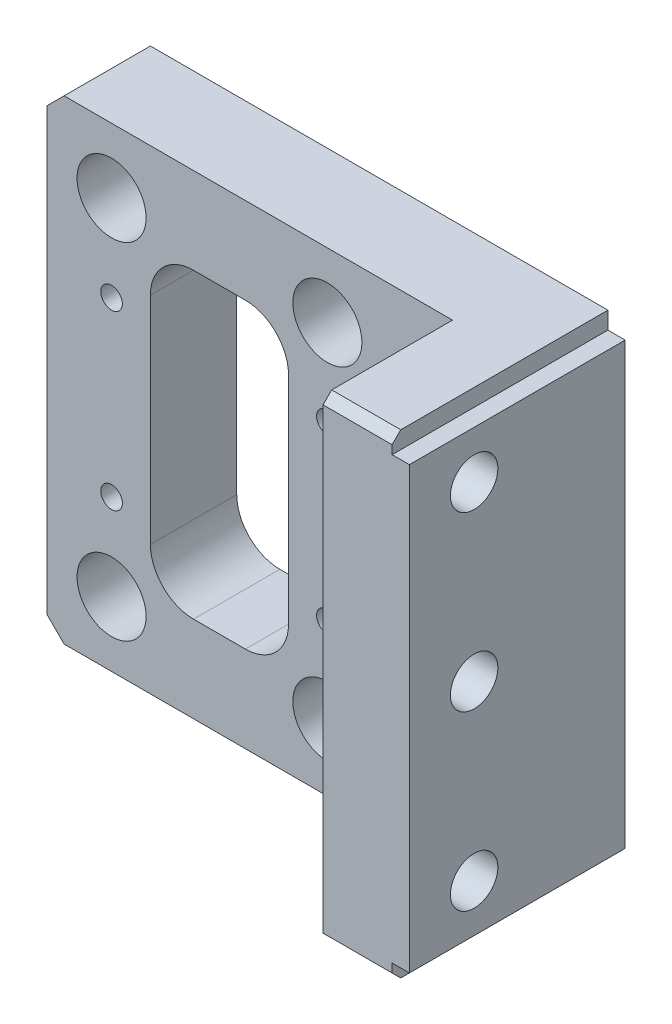
SolidWorks part; units mm, degrees
material "6061-T6 (SS)"
ref_plane "前基準面" through (0, 0, 0) normal (0, 0, 1) x (1, 0, 0)
ref_plane "上基準面" through (0, 0, 0) normal (0, 1, 0) x (1, 0, 0)
ref_plane "右基準面" through (0, 0, 0) normal (1, 0, 0) x (0, 0, -1)
sketch "草图1" plane through (0, 0, 0) normal (0, 0, 1) x (1, 0, 0)
  line L1 (-28.5, -27.5) -> (28.5, -27.5)
  line L2 (-28.5, -27.5) -> (-28.5, 27.5)
  line L3 (-28.5, 27.5) -> (28.5, 27.5)
  line L4 (28.5, -27.5) -> (28.5, 27.5)
  line L5 (-28.5, -27.5) -> (28.5, 27.5) construction
  line L6 (-28.5, 27.5) -> (28.5, -27.5) construction
  point P0 (0, 0)
  dimension "D1" = 57
  dimension "D2" = 55
extrude "凸台-拉伸1" add sketch "草图1" along normal blind 10
sketch "草图2" plane through (0, 0, 10) normal (0, 0, 1) x (1, 0, 0)
  line L0 (-28.5, 27.5) -> (-28.5, -27.5) construction
  line L1 (-16.5, 17.5) -> (-0.5, 17.5)
  line L2 (-16.5, 17.5) -> (-16.5, -17.5)
  line L3 (-16.5, -17.5) -> (-0.5, -17.5)
  line L4 (-0.5, 17.5) -> (-0.5, -17.5)
  line L5 (0, 0) -> (-41.5573, 0) construction
  dimension "D1" = 35
  dimension "D2" = 16
  dimension "D3" = 12
extrude "切除-拉伸1" cut sketch "草图2" against normal through all
hole_wizard "打孔尺寸(%根据)内六角圆柱头螺钉的类型1" positions "草图3" profile "草图4" counterbore size "M4" standard "GB" end condition through all
sketch "草图3" plane through (0, 0, 10) normal (0, 0, 1) x (1, 0, 0)
  line L0 (0, 0) -> (-41.5573, 0) construction
  line L3 (-8.5, -17.5) -> (-8.5, 32.7855) construction
  line L4 (-16.5, -17.5) -> (-0.5, -17.5) construction
  point P0 (-21, 20)
  point P2 (4, 20)
  point P4 (-21, -20)
  point P6 (4, -20)
  dimension "D1" = 40
  dimension "D2" = 25
sketch "草图4" plane through (-21, 20, 10) normal (1, 0, 0) x (0, -1, 0)
  line L0 (0, 0) -> (0, 10)
  line L1 (0, 10) -> (2.4, 10)
  line L3 (2.4, 10) -> (2.4, 6.6)
  line L4 (2.4, 6.6) -> (4, 6.6)
  line L5 (4, 6.6) -> (4, 0)
  line L7 (4, 0) -> (0, 0)
  line L11 (0, -6.35) -> (0, 107.95) construction
  dimension "通孔孔直径" = 4.8
  dimension "通孔孔深度" = 10
  dimension "柱形沉头孔直径" = 8
  dimension "柱形沉头孔深度" = 6.6
hole_wizard "M3 螺纹孔1" positions "草图5" profile "草图6" tap size "M3" standard "GB" end condition through all
sketch "草图5" plane through (0, 0, 10) normal (0, 0, 1) x (1, 0, 0)
  line L0 (-8.5, -17.5) -> (-8.5, 21.3937) construction
  line L1 (-16.5, -17.5) -> (-0.5, -17.5) construction
  line L6 (0, 0) -> (-38.4274, 0) construction
  point P0 (-21, 10)
  point P2 (-21, -10)
  point P4 (4, 10)
  point P6 (4, -10)
  dimension "D1" = 20
  dimension "D2" = 25
cosmetic thread "孔螺蚊线1" parameters "D2"=3
cosmetic thread "孔螺蚊线2" parameters "D2"=3
cosmetic thread "孔螺蚊线3" parameters "D2"=3
cosmetic thread "孔螺蚊线4" parameters "D2"=3
sketch "草图6" plane through (-21, 10, 10) normal (1, 0, 0) x (0, -1, 0)
  line L0 (0, 0) -> (0, 10)
  line L1 (0, 10) -> (1.25, 10)
  line L2 (1.25, 10) -> (1.25, 0)
  line L5 (1.25, 0) -> (0, 0)
  line L11 (0, -6.35) -> (0, 107.95) construction
  dimension "通孔螺纹孔钻头直径" = 2.5
  dimension "通孔螺纹孔钻头深度" = 10
fillet "圆角1" radius 5 4 edges at (-16.5, -17.5, 5) (-0.5, -17.5, 5) (-0.5, 17.5, 5) (-16.5, 17.5, 5)
sketch "草图8" plane through (0, 0, 10) normal (0, 0, 1) x (1, 0, 0)
  line L0 (-28.5, -27.5) -> (28.5, -27.5) construction
  line L1 (28.5, 27.5) -> (18.5, 27.5)
  line L2 (28.5, 27.5) -> (28.5, -27.5)
  line L3 (28.5, -27.5) -> (18.5, -27.5)
  line L4 (18.5, 27.5) -> (18.5, -27.5)
  dimension "D1" = 10
extrude "凸台-拉伸2" add sketch "草图8" along normal blind 15
hole_wizard "打孔尺寸(%根据)内六角圆柱头螺钉的类型2" positions "草图9" profile "草图10" counterbore size "M5" standard "GB" end condition through all
sketch "草图9" plane through (18.5, 0, 0) normal (-1, 0, 0) x (0, 0, 1)
  line L0 (0, 0) -> (27.1852, 0) construction
  line L1 (25, 27.5) -> (25, -27.5) construction
  point P0 (17.5, 20)
  point P2 (17.5, 0)
  point P4 (17.5, -20)
  dimension "D1" = 20
  dimension "D2" = 7.5
sketch "草图10" plane through (18.5, 20, 17.5) normal (0, 1, 0) x (0, 0, 1)
  line L0 (0, 0) -> (0, 10)
  line L1 (0, 10) -> (2.75, 10)
  line L3 (2.75, 10) -> (2.75, 5.7)
  line L4 (2.75, 5.7) -> (5, 5.7)
  line L5 (5, 5.7) -> (5, 0)
  line L7 (5, 0) -> (0, 0)
  line L11 (0, -6.35) -> (0, 107.95) construction
  dimension "通孔孔直径" = 5.5
  dimension "通孔孔深度" = 10
  dimension "柱形沉头孔直径" = 10
  dimension "柱形沉头孔深度" = 5.7
sketch "草图11" plane through (28.5, 0, 0) normal (1, 0, 0) x (0, 0, -1)
  line L0 (0, 0) -> (-29.1646, 0) construction
  line L1 (-25, -27.5) -> (-25, 27.5) construction
  line L2 (0, 27.5) -> (-25, 27.5)
  line L3 (0, 27.5) -> (0, 25.5)
  line L4 (0, 25.5) -> (-25, 25.5)
  line L5 (-25, 27.5) -> (-25, 25.5)
  line L6 (-25, -27.5) -> (-25, -25.5)
  line L7 (0, -25.5) -> (-25, -25.5)
  line L8 (0, -27.5) -> (0, -25.5)
  line L9 (0, -27.5) -> (-25, -27.5)
  line L10 (-25, 27.5) -> (0, 27.5) construction
  line L11 (0, -27.5) -> (0, 27.5) construction
  dimension "D1" = 2
extrude "切除-拉伸2" cut sketch "草图11" against normal blind 2
chamfer "倒角3" distance 2 angle 45 2 edges at (-28.5, -27.5, 5) (-28.5, 27.5, 5)
chamfer "倒角4" distance 1 angle 45 2 edges at (22.5, 27.5, 25) (22.5, -27.5, 25)
